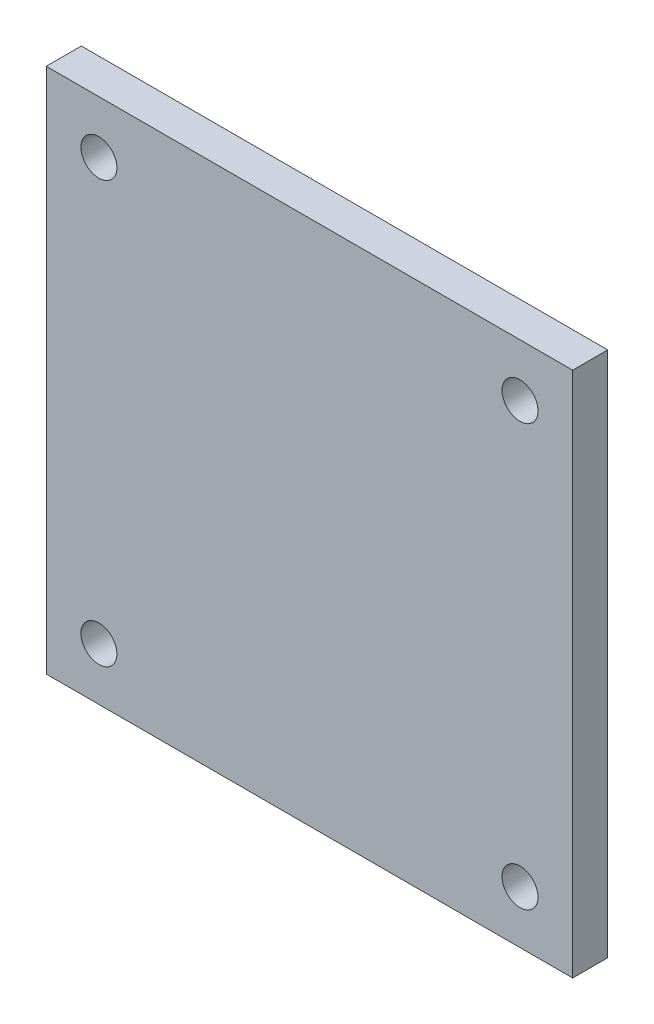
SolidWorks part; units mm, degrees
ref_plane "Front Plane" through (0, 0, 0) normal (0, 0, 1) x (1, 0, 0)
ref_plane "Top Plane" through (0, 0, 0) normal (0, 1, 0) x (1, 0, 0)
ref_plane "Right Plane" through (0, 0, 0) normal (1, 0, 0) x (0, 0, -1)
sketch "Sketch1" plane through (0, 0, 0) normal (0, 0, 1) x (1, 0, 0)
  line L1 (-15, 15) -> (15, 15)
  line L2 (-15, 15) -> (-15, -15)
  line L3 (-15, -15) -> (15, -15)
  line L4 (15, 15) -> (15, -15)
  line L5 (-15, 15) -> (15, -15) construction
  line L6 (-15, -15) -> (15, 15) construction
  point P0 (0, 0)
  dimension "D1" = 30
  dimension "D2" = 30
extrude "Boss-Extrude1" add sketch "Sketch1" along normal blind 2
sketch "Sketch2" plane through (0, 0, 0) normal (0, 0, -1) x (-1, 0, 0)
  line L1 (-15, -15) -> (-15, 15) construction
  line L2 (-15, 15) -> (15, 15) construction
  circle A3 centre (0, 0) radius 6
  dimension "D2" = 15
  dimension "D1" = 15
extrude "Boss-Extrude2" add sketch "Sketch2" along normal blind 8
sketch "Sketch4" plane through (0, 0, 2) normal (0, 0, 1) x (1, 0, 0)
  line L0 (15, 15) -> (-15, 15) construction
  line L3 (-15, 15) -> (-15, -15) construction
  circle A0 centre (-12, 12) radius 0.5
  circle A1 centre (12, 12) radius 0.5
  circle A2 centre (12, -12) radius 0.5
  circle A3 centre (-12, -12) radius 0.5
  dimension "D5" = 1
  dimension "D1" = 3
  dimension "D2" = 3
  dimension "D3" = 2
  dimension "D4" = 2
extrude "Cut-Extrude1" cut sketch "Sketch4" against normal blind 10
sketch "Sketch6" plane through (0, 0, -8) normal (0, 0, -1) x (-1, 0, 0)
  circle A0 centre (0, 0) radius 2.5
  circle A1 centre (0, 0) radius 6 construction
extrude "Cut-Extrude3" cut sketch "Sketch6" against normal blind 9
sketch "Sketch7" plane through (0, 0, 0) normal (0, 1, 0) x (1, 0, 0)
  line L0 (6, 8) -> (-6, 8) construction
  circle A0 centre (0, 5.5) radius 0.5
  dimension "D1" = 2.5
  dimension "D2" = 1
extrude "Cut-Extrude4" cut sketch "Sketch7" along normal blind 0.1 and the other way blind 4
sketch "Sketch8" plane through (0, 0, -8) normal (0, 0, -1) x (-1, 0, 0)
  line L1 (-7.772, 5) -> (7.772, 5)
  line L2 (-7.772, 5) -> (-7.772, -5)
  line L3 (-7.772, -5) -> (7.772, -5)
  line L4 (7.772, 5) -> (7.772, -5)
  line L5 (-7.772, 5) -> (7.772, -5) construction
  line L6 (-7.772, -5) -> (7.772, 5) construction
  point P0 (0, 0)
  dimension "D1" = 10
extrude "Cut-Extrude5" cut sketch "Sketch8" against normal blind 8 flip side to cut
hole_wizard "M3 Tapped Hole1" positions "Sketch9" profile "Sketch10" tap size "M3" standard "GB"
sketch "Sketch9" plane through (0, -5, 0) normal (0, -1, 0) x (-1, 0, 0)
  point P0 (0, 5.5)
sketch "Sketch10" plane through (0, -5, -5.5) normal (1, 0, 0) x (0, 0, -1)
  line L0 (0, 0) -> (0, 3.7511)
  line L1 (0, 3.7511) -> (1.25, 3)
  line L2 (1.25, 3) -> (1.25, 0)
  line L5 (1.25, 0) -> (0, 0)
  line L10 (0, 3.7511) -> (-1.25, 3) construction
  line L11 (0, -6.35) -> (0, 107.95) construction
  dimension "螺纹孔钻头直径" = 2.5
  dimension "螺纹孔钻头深度" = 3
  dimension "导头角度" = 118
cosmetic thread "CosmeticThread1" parameters "D1"=2.8349, "D2"=3
hole_wizard "M2.5 Tapped Hole1" positions "Sketch11" profile "Sketch12" tap size "M2.5" standard "GB" end condition through all
sketch "Sketch11" plane through (0, 0, 2) normal (0, 0, 1) x (1, 0, 0)
  point P0 (12, 12)
  point P3 (12, -12)
  point P6 (-12, -12)
  point P9 (-12, 12)
sketch "Sketch12" plane through (12, 12, 2) normal (1, 0, 0) x (0, -1, 0)
  line L0 (0, 0) -> (0, 10)
  line L1 (0, 10) -> (1.025, 10)
  line L2 (1.025, 10) -> (1.025, 0)
  line L5 (1.025, 0) -> (0, 0)
  line L11 (0, -6.35) -> (0, 107.95) construction
  dimension "通孔螺纹孔钻头直径" = 2.05
  dimension "通孔螺纹孔钻头深度" = 10
cosmetic thread "CosmeticThread2" parameters "D2"=2.5
cosmetic thread "CosmeticThread3" parameters "D2"=2.5
cosmetic thread "CosmeticThread4" parameters "D2"=2.5
cosmetic thread "CosmeticThread5" parameters "D2"=2.5
